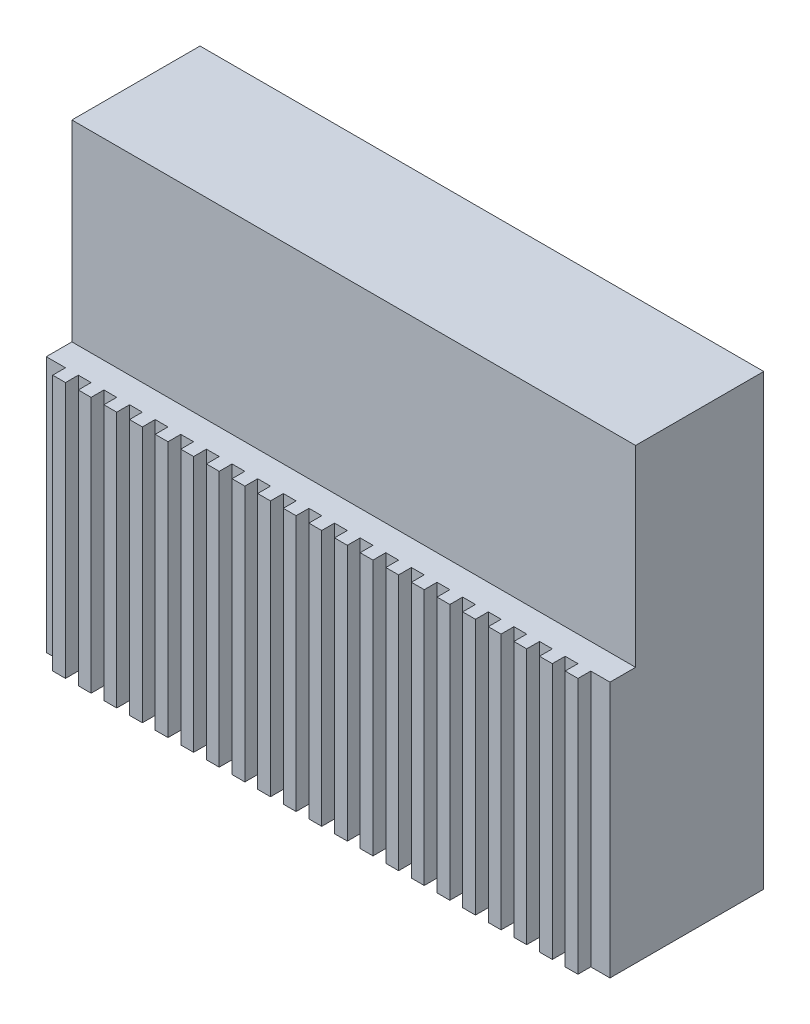
SolidWorks part; units mm, degrees
ref_plane "前视基准面" through (0, 0, 0) normal (0, 0, 1) x (1, 0, 0)
ref_plane "上视基准面" through (0, 0, 0) normal (0, 1, 0) x (1, 0, 0)
ref_plane "右视基准面" through (0, 0, 0) normal (1, 0, 0) x (0, 0, -1)
sketch "草图1" plane through (0, 0, 0) normal (0, 0, 1) x (1, 0, 0)
  line L1 (-22, -17.5) -> (22, -17.5)
  line L2 (-22, -17.5) -> (-22, 17.5)
  line L3 (-22, 17.5) -> (22, 17.5)
  line L4 (22, -17.5) -> (22, 17.5)
  line L5 (-22, -17.5) -> (22, 17.5) construction
  line L6 (-22, 17.5) -> (22, -17.5) construction
  point P0 (0, 0)
  dimension "D1" = 44
  dimension "D2" = 35
extrude "凸台-拉伸1" add sketch "草图1" along normal blind 10
sketch "草图2" plane through (0, 0, 10) normal (0, 0, 1) x (1, 0, 0)
  line L0 (22, -17.5) -> (22, 17.5) construction
  line L1 (-22, -17.5) -> (22, -17.5)
  line L2 (-22, -17.5) -> (-22, 2.5)
  line L3 (-22, 2.5) -> (22, 2.5)
  line L4 (22, -17.5) -> (22, 2.5)
  dimension "D1" = 20
extrude "凸台-拉伸2" add sketch "草图2" along normal blind 2
sketch "草图4" plane through (0, 0, 12) normal (0, 0, 1) x (1, 0, 0)
  line L0 (22, 2.5) -> (-22, 2.5) construction
  line L1 (-0.5, -17.5) -> (0.5, -17.5)
  line L2 (-0.5, -17.5) -> (-0.5, 2.5)
  line L3 (-0.5, 2.5) -> (0.5, 2.5)
  line L4 (0.5, -17.5) -> (0.5, 2.5)
  line L5 (-0.5, -17.5) -> (0.5, 2.5) construction
  line L6 (-0.5, 2.5) -> (0.5, -17.5) construction
  line L7 (-22, -17.5) -> (22, -17.5) construction
  point P0 (0, -7.5)
  point P7 (2.4831, -17.5)
  point P10 (0, 0)
  dimension "D1" = 1
extrude "凸台-拉伸3" add sketch "草图4" along normal blind 1
pattern_linear "阵列(线性)1" count 11 spacing 2 along (1, 0, 0) of "凸台-拉伸3"
mirror "镜向1" about plane through (0, 0, 0) normal (1, 0, 0) of "阵列(线性)1"
